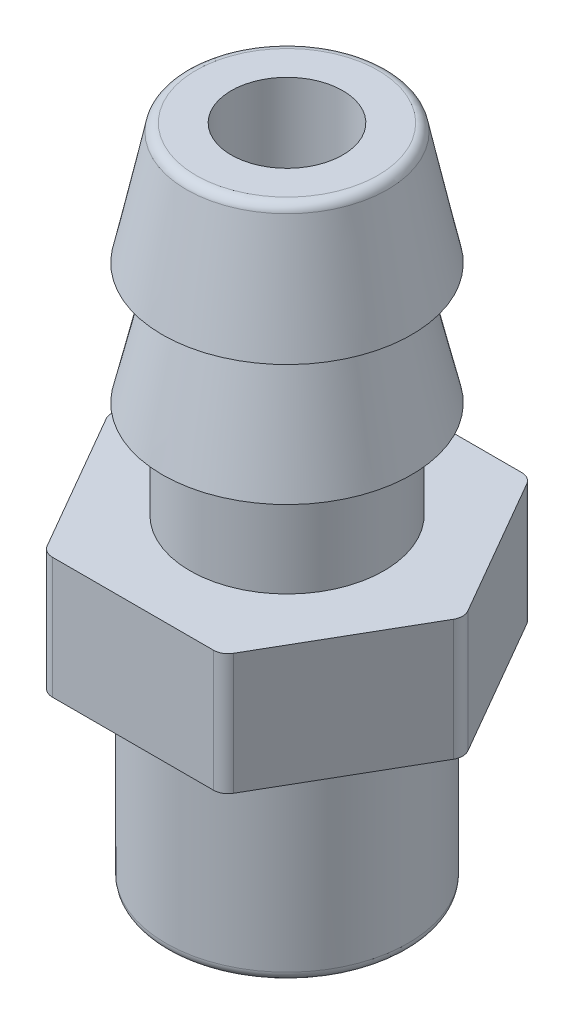
from build123d import *

# Parameters (mm, degrees)
BOSS_EXTRUDE1_DEPTH = 2.5
SKETCH2_R           = 2
BOSS_EXTRUDE2_DEPTH = 2
SKETCH3_R           = 2.57
BOSS_EXTRUDE3_DEPTH = 2.5
BOSS_EXTRUDE3_TAPER = 13
SKETCH4_R           = 2.57
BOSS_EXTRUDE4_DEPTH = 2.5
BOSS_EXTRUDE4_TAPER = 12
SKETCH5_R           = 2.5
SKETCH5_R_2         = 1.15
BOSS_EXTRUDE5_DEPTH = 4.1
SKETCH6_R           = 1.15
CUT_EXTRUDE1_DEPTH  = 11.666370528
FILLET1_R           = 0.3
FILLET2_R           = 0.2


with BuildPart() as part:
    # Sketch1 → Boss-Extrude1 (new body)
    with BuildSketch(Plane(origin=(0, 0, 0), x_dir=(1, 0, 0), z_dir=(0, 1, 0))):
        Polygon((3.666174209, 0), (1.833087105, 3.175), (-1.833087105, 3.175), (-3.666174209, 0), (-1.833087105, -3.175), (1.833087105, -3.175), align=None)
    extrude(amount=BOSS_EXTRUDE1_DEPTH)

    # Sketch2 → Boss-Extrude2 (add)
    with BuildSketch(Plane(origin=(0, 2.5, 0), x_dir=(1, 0, 0), z_dir=(0, 1, 0))):
        with Locations(Location((0, 0, 0), (0, 0, 270))):
            Circle(SKETCH2_R)
    extrude(amount=BOSS_EXTRUDE2_DEPTH)

    # Sketch3 → Boss-Extrude3 (add)
    with BuildSketch(Plane(origin=(0, 4.5, 0), x_dir=(1, 0, 0), z_dir=(0, 1, 0))):
        Circle(SKETCH3_R)
    extrude(amount=BOSS_EXTRUDE3_DEPTH, taper=BOSS_EXTRUDE3_TAPER)

    # Sketch4 → Boss-Extrude4 (add)
    with BuildSketch(Plane(origin=(0, 7, 0), x_dir=(1, 0, 0), z_dir=(0, 1, 0))):
        Circle(SKETCH4_R)
    extrude(amount=BOSS_EXTRUDE4_DEPTH, taper=BOSS_EXTRUDE4_TAPER)

    # Sketch5 → Boss-Extrude5 (add)
    with BuildSketch(Plane.XZ):
        with Locations(Location((0, 0, 0), (0, 0, 90))):
            Circle(SKETCH5_R)
        with Locations(Location((0, 0, 0), (0, 0, 270))):
            Circle(SKETCH5_R_2, mode=Mode.SUBTRACT)
    extrude(amount=BOSS_EXTRUDE5_DEPTH)

    # Sketch6 → Cut-Extrude1 (cut, through all)
    with BuildSketch(Plane.XZ):
        with Locations(Location((0, 0, 0), (0, 0, 270))):
            Circle(SKETCH6_R)
    extrude(amount=-CUT_EXTRUDE1_DEPTH, mode=Mode.SUBTRACT)

    # Fillet1
    fillet1_edges = [part.edges().sort_by_distance(p)[0] for p in [
        (1.833087105, 1.25, 3.175),
        (-1.833087105, 1.25, 3.175),
        (-3.666174209, 1.25, 0),
        (-1.833087105, 1.25, -3.175),
        (1.833087105, 1.25, -3.175),
        (3.666174209, 1.25, 0),
    ]]
    fillet(fillet1_edges, radius=FILLET1_R)

    # Fillet2
    fillet2_edges = [part.edges().sort_by_distance(p)[0] for p in [
        (-2.038608596, 9.5, 0),
        (0, -4.1, -2.5),
    ]]
    fillet(fillet2_edges, radius=FILLET2_R)


solid = part.part
